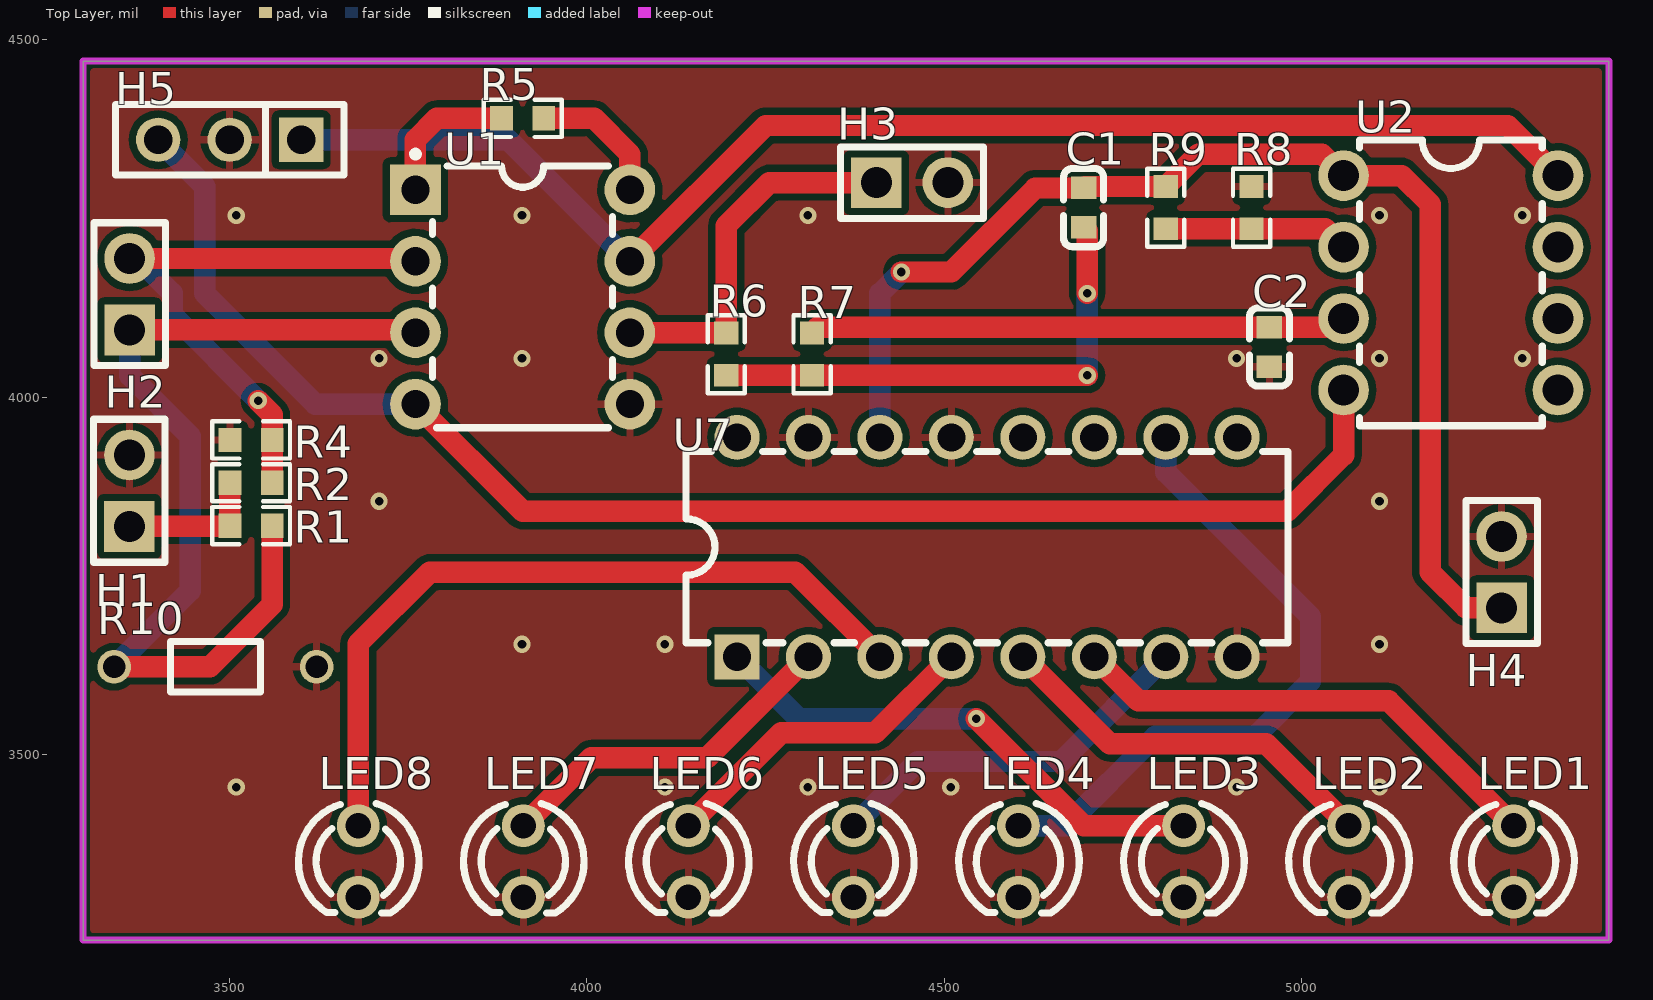
[diagram p0: Top Layer view]
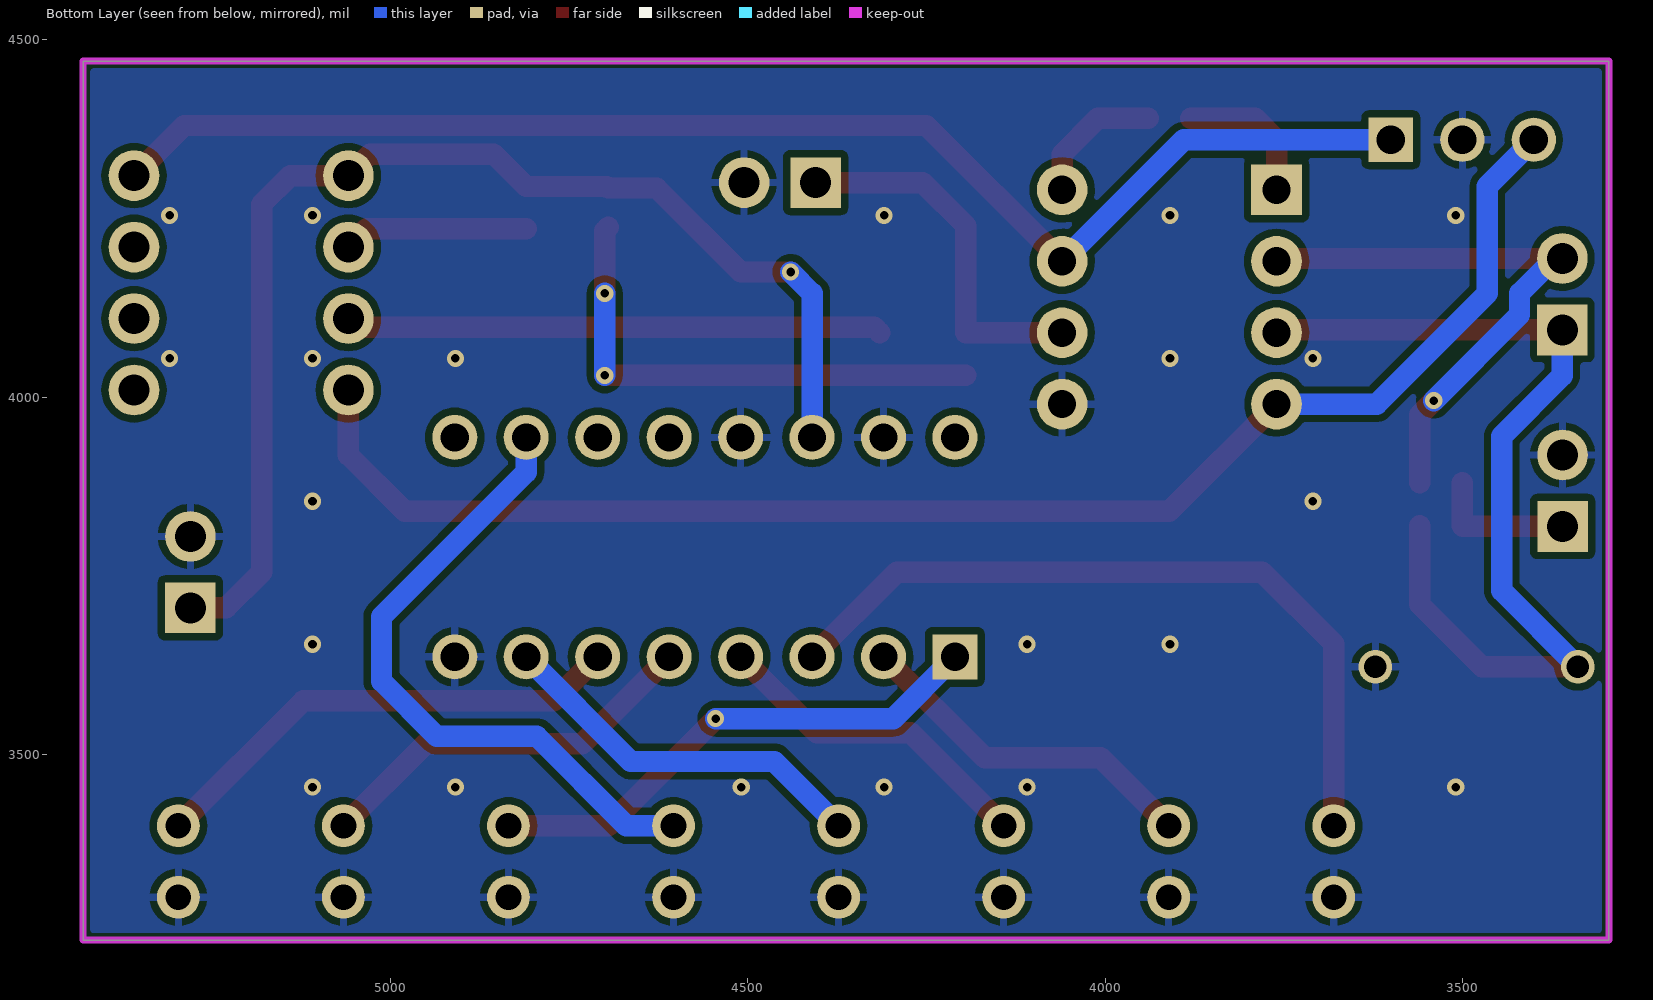
[diagram p1: Bottom Layer view, seen from below]
# Altium PCB MISC51786.pcbdoc
Units mil, origin at the board's own origin, x right, y up, seen from the top; angles counter-clockwise.
Board outline 2135 x 1230 mil, 2 copper layers (Top Layer, Bottom Layer), stack 62.206 mil thick; 27 components, 22 nets, 81 pads, 26 vias.

## Layer stack, top to bottom
Top Solder Mask Layer: solder mask 0.394, Dk 3.3
Top Layer: signal copper 1.379
Dielectric1: surface 59.449, FR4, Dk 4.5
Bottom Layer: signal copper 1.378
Bottom Solder Mask Layer: solder mask 0.394, Dk 3.3

## Board outline
3295,4470 3295,3240 5430,3240 5430,4470

## Design rules (kind name [scope] priority, off if disabled: settings)
BoardOutlineClearance copperThickness2oz_1 [All] p2 off: genericclearance=7.99 ignorepadtopadclearanceinfootprint=FALSE except(0: Arc-SplitContinuation Track-SplitContinuation SMDPad-SplitContinuation THPad-SplitContinuation Via-SplitContinuation Fill-SplitContinuation Region-SplitContinuation Poly-SplitContinuation Text-SplitContinuation Hole-SplitContinuation; 5.98: Arc-CutoutEdge SMDPad-CutoutEdge THPad-CutoutEdge Via-CutoutEdge Fill-CutoutEdge Region-CutoutEdge Text-CutoutEdge; 6.93: Hole-OutlineEdge Hole-CutoutEdge; 10: Poly-OutlineEdge Poly-CutoutEdge; 11.81: Arc-OutlineEdge Track-OutlineEdge SMDPad-OutlineEdge THPad-OutlineEdge Via-OutlineEdge Fill-OutlineEdge Region-OutlineEdge Text-OutlineEdge Track-CutoutEdge)
BoardOutlineClearance copperThickness1oz_1 [All] p4: genericclearance=4.02 ignorepadtopadclearanceinfootprint=FALSE except(0: Arc-SplitContinuation Track-SplitContinuation SMDPad-SplitContinuation THPad-SplitContinuation Via-SplitContinuation Fill-SplitContinuation Region-SplitContinuation Poly-SplitContinuation Text-SplitContinuation Hole-SplitContinuation; 6: SMDPad-CutoutEdge THPad-CutoutEdge Via-CutoutEdge Fill-CutoutEdge Region-CutoutEdge Text-CutoutEdge; 6.93: Hole-OutlineEdge Hole-CutoutEdge; 10: Poly-OutlineEdge Poly-CutoutEdge; 11.8: Arc-OutlineEdge Track-OutlineEdge SMDPad-OutlineEdge THPad-OutlineEdge Via-OutlineEdge Fill-OutlineEdge Region-OutlineEdge Text-OutlineEdge; 11.81: Arc-CutoutEdge Track-CutoutEdge)
Clearance copperThickness2oz [All] p1 off: gap=7.99 ignorepadtopadclearanceinfootprint=FALSE except(5.98: SMDPad-Track SMDPad-SMDPad THPad-Track SMDPad-THPad THPad-THPad Track-Via SMDPad-Via THPad-Via Via-Via Fill-Track Region-Track Fill-SMDPad Region-SMDPad Fill-THPad Region-THPad Fill-Via Region-Via Fill-Fill Fill-Region Region-Region Arc-Track Arc-SMDPad Arc-THPad Arc-Via Fill-Arc Region-Arc Arc-Arc Text-Track SMDPad-Text Text-THPad Text-Via Fill-Text Region-Text Arc-Text Text-Text; 6.93: Hole-Track Hole-SMDPad Hole-THPad Hole-Via Fill-Hole Region-Hole Hole-Arc Hole-Text; 10: Poly-Track Poly-SMDPad Poly-THPad Poly-Via Poly-Fill Poly-Region Poly-Poly Poly-Arc Poly-Text Poly-Hole)
Clearance copperThickness1oz [All] p3: gap=4.02 ignorepadtopadclearanceinfootprint=FALSE except(5.98: SMDPad-Track SMDPad-SMDPad THPad-Track SMDPad-THPad THPad-THPad Track-Via SMDPad-Via THPad-Via Via-Via Fill-Track Region-Track Fill-SMDPad Region-SMDPad Fill-THPad Region-THPad Fill-Via Region-Via Fill-Fill Fill-Region Region-Region; 6: Arc-Track Arc-SMDPad Arc-THPad Arc-Via Fill-Arc Region-Arc Arc-Arc Text-Track SMDPad-Text Text-THPad Text-Via Fill-Text Region-Text Arc-Text Text-Text; 6.93: Hole-Track Hole-SMDPad Hole-THPad Hole-Via Fill-Hole Region-Hole Hole-Arc Hole-Text; 10: Poly-Track Poly-SMDPad Poly-THPad Poly-Via Poly-Fill Poly-Region Poly-Poly Poly-Arc Poly-Text Poly-Hole)
DiffPairsRouting differentialPair [All] p1: maxlimit=6 minlimit=6 mostfreqgap=6 toplayer_minwidth=5 toplayer_prefwidth=10 toplayer_maxwidth=100 toplayer_mingap=6 toplayer_prefgap=6 toplayer_maxgap=6 bottomlayer_minwidth=5 bottomlayer_prefwidth=10 bottomlayer_maxwidth=100 bottomlayer_mingap=6 bottomlayer_prefgap=6 bottomlayer_maxgap=6 maxuncoupledlength=10
HoleToHoleClearance otherClearance [All] p1: gap=11.81 allowstackedmicrovias=TRUE
Length netLength [All] p1: minlimit=0 maxlimit=0
MatchedLengths netLengthTolerance [All] p1: tolerance=1000
PasteMaskExpansion pasteMaskExpansion [All] p1: expansion=0
PlaneConnect innerPlane [All] p1: planeconnectstyle=Relief reliefexpansion=20 reliefentries=4 reliefconductorwidth=10 reliefairgap=10
PolygonConnect copperRegion [(InNet('GND'))] p1: connectstyle=Relief reliefconductorwidth=10 reliefentries=4 polygonreliefangle="90 Angle" airgapwidth=10 via.connectstyle=Relief via.reliefconductorwidth=10 via.reliefentries=4 via.polygonreliefangle="90 Angle" via.airgapwidth=10
RoutingVias viaSize [All] p1: holewidth=12.01 width=24.02 viastyle="Through Hole" minholewidth=11.81 minwidth=19.68 maxholewidth=248.03 maxwidth=393.7
SolderMaskExpansion solderMaskExpansion [IsVia] p1: expansion=-1000 istentingtop=TRUE
SolderMaskExpansion solderMaskExpansion [All] p2: expansion=2 istentingtop=FALSE
Width copperThickness2oz_2 [All] p1 off: maxlimit=100 minlimit=8 preferedwidth=10
Width copperThickness1oz_2 [All] p2: maxlimit=100 minlimit=5 preferedwidth=10

## Components (designator, comment, footprint, x,y, rotation, side; value= is the part's Value field where it differs from the comment)
C1 "1.6uF" C0603 4695,4265 r90 top
C2 "1.6uF" C0603 4955,4070 r90 top
H1 "" HDR-TH_2P-P2.54-V-M-1 3359.68,3868.88 r90 top
H2 "" HDR-TH_2P-P2.54-V-M-1 3360,4143.88 r90 top
H3 "" HDR-TH_2P-P2.54-V-M-1 4455,4300 r0 top
H4 "" HDR-TH_2P-P2.54-V-M-1 5280,3755 r90 top
H5 "" HDR-TH_3P-P2.54-V-F 3500,4360 r180 top
LED1 "" LED_TH-3mm 5296.76,3350 r270 top
LED2 "" LED_TH-3mm 5065.8,3350 r270 top
LED3 "" LED_TH-3mm 4834.83,3350 r270 top
LED4 "" LED_TH-3mm 4603.86,3350 r270 top
LED5 "" LED_TH-3mm 4372.9,3350 r270 top
LED6 "" LED_TH-3mm 4141.93,3350 r270 top
LED7 "" LED_TH-3mm 3910.97,3350 r270 top
LED8 "" LED_TH-3mm 3680,3350 r270 top
R1 "1K" R0603 3530,3820 r0 top
R2 "1K" R0603 3530,3880 r0 top
R4 "1K" R0603 3530,3940 r180 top
R5 "5.49kΩ" R0603 3910,4390 r0 top
R6 "1.5K" R0603 4195,4060 r90 top
R7 "1.5K" R0603 4315,4060 r270 top
R8 "10K" R0603 4930,4265 r270 top
R9 "10K" R0603 4810,4265 r270 top
R10 "10kΩ" Res_1/8W 3480,3620 r0 top
U1 "AD620AN" DIP-8_L9.3-W6.4-P2.54-LS7.6-BL 3910,4140 r270 top
U2 "741" PDIP-8_L10.2-W6.5-P2.54-LS7.6-BL 5208.83,4159.75 r270 top
U7 "CD40175BF3A" CDIP-16_L21.4-W6.8-P2.54-LS7.8-BL 4560,3790 r0 top

## Footprints (in the part's own frame and the unit in brackets; to place one, negate y for a bottom-side part, rotate by r counter-clockwise, add the part's x,y. Pads: shape width x height; smd on the part's side, far side on the other; paste and mask are expansions set on the pad)
C0603 [mm]
  rect 0.8x0.9 smd: 1(-0.7,0) 2(0.7,0)
  silkscreen extent -1.39,-0.71 1.39,0.71
CDIP-16_L21.4-W6.8-P2.54-LS7.8-BL [mm]
  rect 1.6x1.6 hole 1: 1(-8.89,-3.9)
  round 1.6 hole 1 copper offset 0,0: 2(-6.35,-3.9) 3(-3.81,-3.9) 4(-1.27,-3.9) 5(1.27,-3.9) 6(3.81,-3.9) 7(6.35,-3.9) 8(8.89,-3.9) 9(8.89,3.9) 10(6.35,3.9) 11(3.81,3.9) 12(1.27,3.9) 13(-1.27,3.9) 14(-3.81,3.9) 15(-6.35,3.9) 16(-8.89,3.9)
  silkscreen extent -10.7,-3.4 10.7,3.4
DIP-8_L9.3-W6.4-P2.54-LS7.6-BL [mm]
  rect 1.8x1.8 hole 1: 1(-3.81,-3.81)
  round 1.8 hole 1: 2(-1.27,-3.81) 3(1.27,-3.81) 4(3.81,-3.81) 5(3.81,3.81) 6(1.27,3.81) 7(-1.27,3.81) 8(-3.81,3.81)
  silkscreen extent -5.18,-3.91 4.65,3.2
HDR-TH_2P-P2.54-V-M-1 [mm]
  rect 1.8x1.8 hole 1.1: 1(-1.27,0)
  round 1.8 hole 1.1: 2(1.27,0)
  silkscreen extent -2.54,-1.27 2.54,1.27
HDR-TH_3P-P2.54-V-F [mil]
  rect 62x62 hole 40.16: 1(-100,0)
  round 62 hole 40.16: 2(0,0) 3(100,0)
  silkscreen extent -160,-49 160,49
LED_TH-3mm [mil]
  round 60 hole 36 paste+0 mask+2: 1(-50,0) 2(50,0)
  silkscreen extent -81,-84 72,85
PDIP-8_L10.2-W6.5-P2.54-LS7.6-BL [mm]
  round 1.8 hole 1.1: 1(-3.81,-3.81) 2(-1.27,-3.81) 3(1.27,-3.81) 4(3.81,-3.81) 5(3.81,3.81) 6(1.27,3.81) 7(-1.27,3.81) 8(-3.81,3.81)
  silkscreen extent -5.08,-3.25 5.08,3.25
R0603 [mil]
  rect 31.75x34.02 smd paste-3937.01 mask+2: 1(-29.66,0) 2(29.66,0)
  silkscreen extent -55,-26 55,26
Res_1/8W [mil]
  round 47.2 hole 31.5 paste+0 mask+2: 1(-141.7,2.48) 2(141.7,2.48)
  silkscreen extent -63,-33 63,38

## Via types
v1: diameter 24.02, hole 12, Top Layer to Bottom Layer, 26 vias

## Nets (pads, with @x,y where several pads share a name; then routed paths per layer and width w, separated by ;. In a path a pad name is that pad's centre, name@x,y a point inside that pad or via, vN(x,y) a via of type N, cw(c..) or ccw(c..) an arc to the next point about the centre after c; other vN are vias at no path point)
12V: H5.1 U1.7 U2.8 | length 1937
  Top Layer w30: U1.7 4250,4380 5288.59,4380 U2.8
  Bottom Layer w30: H5.1 3890,4360 U1.7
$1N1: H1.1 R1.1 R2.1 | length 201.1
  Top Layer w30: H1.1 3499.22,3818.88 R1.1 R2.1
$1N6: H2.2 R2.2 R4.1 U1.2 | length 804.7
  Top Layer w30: H2.2 3756.12,4193.88 U1.2 ; v1(3540,3995) 3559.66,3975.34 R4.1 R2.2
  Bottom Layer w30: H2.2 3371.12,4193.88 3420,4145 3420,4115 v1(3540,3995)
$1N8: H2.1 R1.2 R10.1 U1.3 | length 1320.2
  Top Layer w30: R10.1 3472.48,3622.48 3559.66,3709.66 R1.2 ; H2.1 3756.12,4093.88 U1.3
  Bottom Layer w30: R10.1 3445,3729.18 3445,3945 3360,4030 H2.1
$1N13: H3.1 R6.2 U1.6 | length 520.3
  Top Layer w30: U1.6 4060.34,4089.66 R6.2 4195,4240 4255,4300 H3.1
$1N14: R5.1 U1.1 | length 202.8
  Top Layer w30: U1.1 3760,4360 3790,4390 R5.1
$1N15: R5.2 U1.8 | length 191.1
  Top Layer w30: R5.2 4010,4390 4060,4340 U1.8
$1N17: C1.1 R6.1 R7.2 | length 714.2
  Top Layer w30: R6.1 R7.2 v1(4700,4030.34) ; C1.1 4700,4232.44 v1(4700,4145)
  Bottom Layer w30: v1(4700,4030.34) v1(4700,4145)
$1N18: C2.2 R7.1 U2.3 | length 752.2
  Top Layer w30: R7.1 4322.9,4097.56 C2.2 5046.64,4097.56 U2.3
$1N21: R8.2 R9.2 U2.2 | length 259.4
  Top Layer w30: R9.2 R8.2 5033.25,4235.34 U2.2
$1N35: C1.2 H4.1 R9.1 U2.1 U7.14 | length 1716.9
  Top Layer w30: v1(4440,4175) 4510,4175 4627.56,4292.56 C1.2 4697.1,4294.66 R9.1 4855.34,4340 5028.59,4340 U2.1 5140.25,4309.75 5180,4270 5180,3755 5230,3705 H4.1
  Bottom Layer w30: U7.14@4410,3943.54 4410,4145 v1(4440,4175)
$1N43: LED6.1 U7.4 | length 466
  Top Layer w30: LED6.1 4271.93,3530 4403.54,3530 U7.4
$1N44: LED5.1 U7.7 | length 535
  Bottom Layer w30: LED5.1 4462.9,3490 4663.54,3490 U7.7
$1N45: LED4.1 U7.10 | length 917.4
  Bottom Layer w30: LED4.1 4670,3400 4795,3525 4935,3525 5012.5,3602.5 5012.5,3692.5 4810,3895 U7.10@4810,3943.54
$1N46: LED3.1 U7.1 | length 722.8
  Top Layer w30: v1(4545,3550) 4695,3400 LED3.1
  Bottom Layer w30: U7.1 4296.46,3550 v1(4545,3550)
$1N47: LED2.1 U7.5 | length 553.7
  Top Layer w30: U7.5 4731.46,3515 4950.8,3515 LED2.1
$1N48: LED1.1 U7.6 | length 684.7
  Top Layer w30: U7.6 4771.46,3575 5121.76,3575 LED1.1
$1N49: LED7.1 U7.2 | length 497
  Top Layer w30: LED7.1 4005.97,3495 4168.54,3495 U7.2
$1N50: LED8.1 U7.3 | length 1075.5
  Top Layer w30: LED8.1 3680,3655 3780,3755 4291.46,3755 U7.3
-12V: H5.3 U1.4 U2.4 | length 2085.7
  Top Layer w30: U1.4 3910,3840 4980,3840 5058.83,3918.83 U2.4
  Bottom Layer w30: H5.3 3465,4295 3465,4145 3620,3990 U1.4
GND: C2.1 H1.2 H3.2 H4.2 H5.2 LED1.2 LED2.2 LED3.2 LED4.2 LED5.2 LED6.2 LED7.2 LED8.2 R4.2 R8.1 R10.2 U1.5 U7.8 U7.13 U7.15
  other v1: 3509.1,3454.1 4109.1,3454.1 4309.1,3454.1 4509.1,3454.1 4909.1,3454.1 5109.1,3454.1 3909.1,3654.1 4109.1,3654.1 5109.1,3654.1 3709.1,3854.1 5109.1,3854.1 3709.1,4054.1 3909.1,4054.1 4909.1,4054.1 5109.1,4054.1 5309.1,4054.1 3509.1,4254.1 3909.1,4254.1 4309.1,4254.1 5109.1,4254.1 5309.1,4254.1
VCC: U7.16
pads on no net: U2.5 U2.6 U2.7 U7.9 U7.11 U7.12

## Polygon pours and split planes (outlines as drawn)
GND on Bottom Layer (solid, remove dead copper, pour order 2): 3000,4575 3000,3105 5580,3105 5580,4575
GND on Top Layer (solid, remove dead copper, pour order 2): 3110,4555 3110,3000 5600,3000 5600,4555

## Keep-outs
Board Outline Layer:
  the board outline again, w10